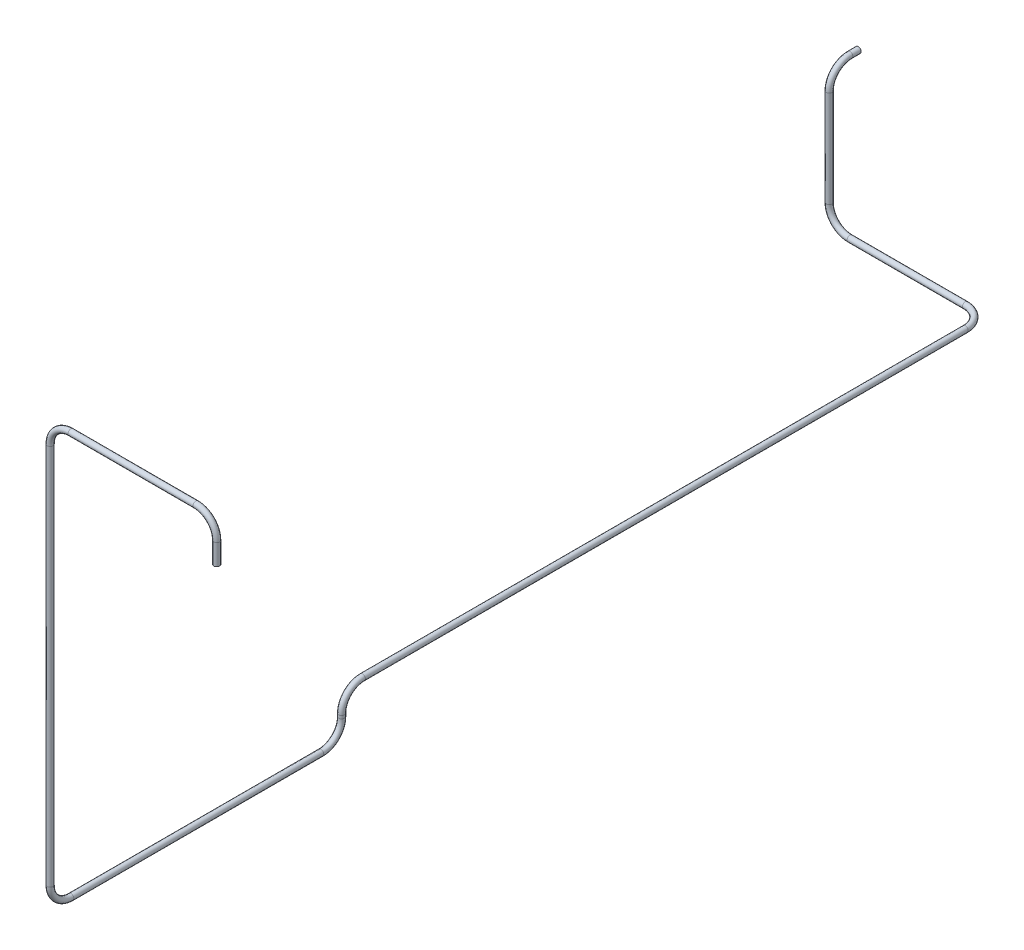
SolidWorks part; units mm, degrees
ref_plane "Front Plane" through (0, 0, 0) normal (0, 0, 1) x (1, 0, 0)
ref_plane "Top Plane" through (0, 0, 0) normal (0, 1, 0) x (1, 0, 0)
ref_plane "Right Plane" through (0, 0, 0) normal (1, 0, 0) x (0, 0, -1)
sketch "Sketch 1" plane through (0, 0, 0) normal (0, 0, 1) x (1, 0, 0)
  line L0 (0, 208.6331) -> (0, -141.7266) construction
  line L1 (-142.446, 0) -> (127.3381, 0) construction
  line L2 (200, 0) -> (200, 50)
  line L3 (150, 100) -> (-150, 100)
  line L4 (-200, 50) -> (-200, -816.5)
  arc A0 (-150, 100) -> (-200, 50) centre (-150, 50) ccw
  arc A1 (200, 50) -> (150, 100) centre (150, 50) ccw
  point P13 (-200, 100)
  point P16 (200, 100)
  dimension "D3" = 50
  dimension "D1" = 100
  dimension "D2" = 400
  dimension "D4" = 816.5
sketch "Sketch 2" plane through (0, 0, 0) normal (0, 1, 0) x (1, 0, 0)
  circle A0 centre (200, 0) radius 4
  circle A1 centre (200, 0) radius 7
  dimension "D1" = 8
  dimension "D2" = 3
sweep "Sweep 1" add profiles "Sketch 2" path "Sketch 1"
ref_plane "Plane 1" through (-200, 0, 0) normal (1, 0, 0) x (0, 0, -1)
sketch "Sketch 3" plane through (-200, 0, 0) normal (1, 0, 0) x (0, 0, -1)
  line L0 (0, -816.5) -> (0, -866.5)
  line L1 (-7, -816.5) -> (7, -816.5) construction
  line L2 (50, -916.5) -> (650, -916.5)
  line L3 (700, -866.5) -> (700, -859.5)
  line L4 (750, -809.5) -> (2147.5, -809.5)
  arc A0 (700, -859.5) -> (750, -809.5) centre (750, -859.5) cw
  arc A1 (650, -916.5) -> (700, -866.5) centre (650, -866.5) ccw
  arc A2 (0, -866.5) -> (50, -916.5) centre (50, -866.5) ccw
  point P10 (700, -809.5)
  point P13 (700, -916.5)
  point P16 (0, -916.5)
  dimension "D3" = 50
  dimension "D1" = 100
  dimension "D2" = 107
  dimension "D4" = 750
  dimension "D5" = 1397.5
sketch "Sketch 4" plane through (0, -816.5, 0) normal (0, -1, 0) x (1, 0, 0)
  circle A0 centre (-200, 0) radius 4 construction
  circle A1 centre (-200, 0) radius 7
  circle A2 centre (-200, 0) radius 7
  circle A3 centre (-200, 0) radius 4
  dimension "D1" = 0
sweep "Sweep 2" add profiles "Sketch 4" path "Sketch 3"
ref_plane "Plane 2" through (0, -809.5, 0) normal (0, 1, 0) x (1, 0, 0)
sketch "Sketch 5" plane through (0, -809.5, 0) normal (0, 1, 0) x (1, 0, 0)
  line L0 (-200, 2147.5) -> (-200, 2197.5)
  line L1 (-193, 2147.5) -> (-207, 2147.5) construction
  line L2 (-449.9, 2247.5) -> (-250, 2247.5)
  arc A0 (-250, 2247.5) -> (-200, 2197.5) centre (-250, 2197.5) cw
  point P7 (-200, 2247.5)
  point P12 (-200, 2247.5)
  dimension "D2" = 50
  dimension "D1" = 100
  dimension "D3" = 249.9
sketch "Sketch 6" plane through (0, 0, -2147.5) normal (0, 0, -1) x (-1, 0, 0)
  circle A0 centre (200, -809.5) radius 4 construction
  circle A1 centre (200, -809.5) radius 7
  circle A2 centre (200, -809.5) radius 7
  circle A3 centre (200, -809.5) radius 4
  dimension "D1" = 0
sweep "Sweep 3" add profiles "Sketch 6" path "Sketch 5"
ref_plane "Plane 3" through (0, 0, -2247.5) normal (0, 0, 1) x (1, 0, 0)
sketch "Sketch 7" plane through (0, 0, -2247.5) normal (0, 0, 1) x (1, 0, 0)
  line L0 (-526.9371, -809.5) -> (-449.9, -809.5)
  line L2 (-576.9371, -759.5) -> (-576.9371, -577.5)
  line L3 (-449.9, -802.5) -> (-449.9, -816.5) construction
  arc A0 (-576.9371, -759.5) -> (-526.9371, -809.5) centre (-526.9371, -759.5) ccw
  point P7 (-576.9371, -809.5)
  dimension "D3" = 77.0371
  dimension "D2" = 50
  dimension "D1" = 232
sketch "Sketch 8" plane through (-449.9, 0, 0) normal (-1, 0, 0) x (0, 0, 1)
  circle A0 centre (-2247.5, -809.5) radius 4 construction
  circle A1 centre (-2247.5, -809.5) radius 7
  circle A2 centre (-2247.5, -809.5) radius 7
  circle A3 centre (-2247.5, -809.5) radius 4
  dimension "D1" = 0
sweep "Sweep 4" add profiles "Sketch 8" path "Sketch 7"
ref_plane "Plane 4" through (-576.9371, 0, 0) normal (1, 0, 0) x (0, 0, -1)
sketch "Sketch 9" plane through (-576.9371, 0, 0) normal (1, 0, 0) x (0, 0, -1)
  line L0 (2247.5, -577.5) -> (2247.5, -527.5)
  line L1 (2254.5, -577.5) -> (2240.5, -577.5) construction
  line L2 (2297.5, -477.5) -> (2317.5, -477.5)
  arc A0 (2247.5, -527.5) -> (2297.5, -477.5) centre (2297.5, -527.5) cw
  point P7 (2247.5, -477.5)
  dimension "D2" = 50
  dimension "D1" = 100
  dimension "D3" = 20
sketch "Sketch 10" plane through (0, -577.5, 0) normal (0, 1, 0) x (1, 0, 0)
  circle A0 centre (-576.9371, 2247.5) radius 4 construction
  circle A1 centre (-576.9371, 2247.5) radius 7
  circle A2 centre (-576.9371, 2247.5) radius 7
  circle A3 centre (-576.9371, 2247.5) radius 4
  dimension "D1" = 0
sweep "Sweep 5" add profiles "Sketch 10" path "Sketch 9"
